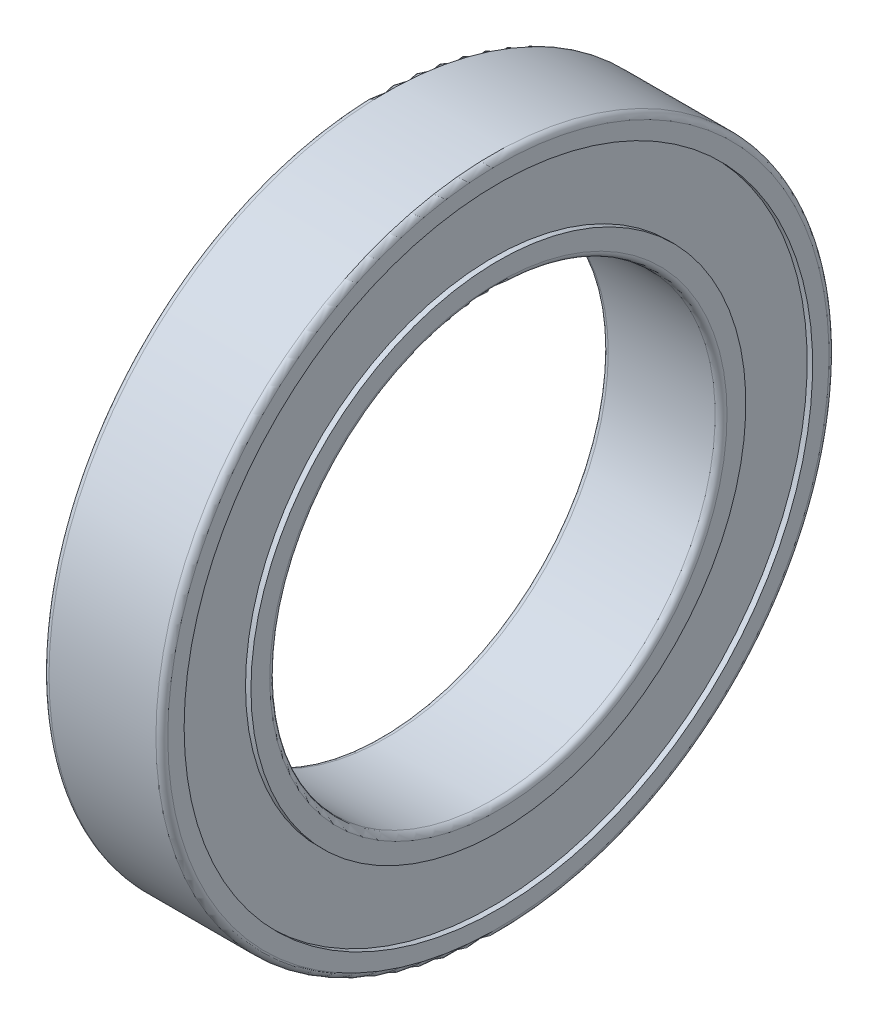
from build123d import *

# Parameters (mm, degrees)
FILLET1_R = 0.6
FILLET2_R = 0.6


with BuildPart() as part:
    # Sketch1 → Revolve1 (revolve)
    with BuildSketch(Plane.XY, mode=Mode.PRIVATE) as revolve1_sk:
        Polygon((0, 22.5), (12, 22.5), (12, 25), (11.45, 25), (11.45, 31.75), (12, 31.75), (12, 34), (0, 34), (0, 31.75), (0.55, 31.75), (0.55, 25), (0, 25), align=None)
    revolve(revolve1_sk.sketch.rotate(Axis((0, 0, 0), (1, 0, 0)), 90), axis=Axis((0, 0, 0), (1, 0, 0)))

    # Fillet1
    fillet1_edges = [part.edges().sort_by_distance(p)[0] for p in [
        (0, 0, -34),
        (12, 0, -34),
    ]]
    fillet(fillet1_edges, radius=FILLET1_R)

    # Fillet2
    fillet2_edges = [part.edges().sort_by_distance(p)[0] for p in [
        (12, 0, -22.5),
        (0, 0, -22.5),
    ]]
    fillet(fillet2_edges, radius=FILLET2_R)


solid = part.part
